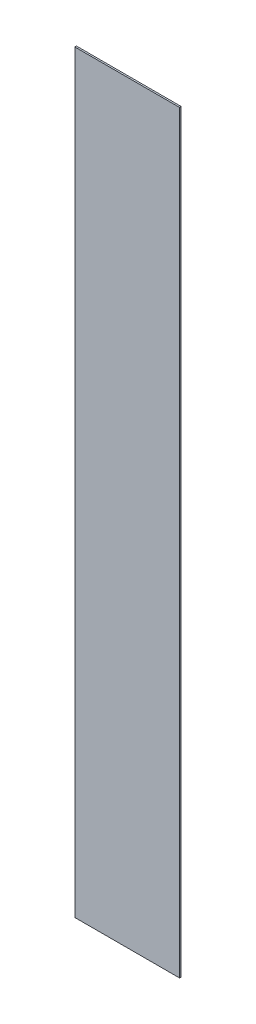
SolidWorks part; units mm, degrees
material "PMMA(有机玻璃)"
ref_plane "前视" through (0, 0, 0) normal (0, 0, 1) x (1, 0, 0)
ref_plane "上视" through (0, 0, 0) normal (0, 1, 0) x (1, 0, 0)
ref_plane "右视" through (0, 0, 0) normal (1, 0, 0) x (0, 0, -1)
sketch "草图1" plane through (0, 0, 0) normal (0, 0, 1) x (1, 0, 0)
  line L1 (-160.5, 1155) -> (160.5, 1155)
  line L2 (-160.5, 1155) -> (-160.5, -1155)
  line L3 (-160.5, -1155) -> (160.5, -1155)
  line L4 (160.5, 1155) -> (160.5, -1155)
  line L5 (-160.5, 1155) -> (160.5, -1155) construction
  line L6 (-160.5, -1155) -> (160.5, 1155) construction
  point P0 (0, 0)
  dimension "D1" = 2310
  dimension "D2" = 321
extrude "凸台-拉伸1" add sketch "草图1" along normal blind 5
hole_wizard "M5 间隙孔1" positions "草图3" profile "草图2" hole size "M5" standard "GB"
sketch "草图3" plane through (0, 0, 5) normal (0, 0, 1) x (1, 0, 0)
  line L0 (-427.5, 273) -> (-427.5, -273) construction
  line L1 (-427.5, -273) -> (427.5, -273) construction
  line L2 (0, 273) -> (0, -273) construction
  line L3 (427.5, 273) -> (-427.5, 273) construction
  line L5 (-427.5, 0) -> (427.5, 0) construction
  line L6 (427.5, -273) -> (427.5, 273) construction
  point P0 (-375, -261)
  point P46 (415.5, 250)
  point P48 (-415.5, 250)
  point P58 (-125, -261)
  point P59 (125, -261)
  point P61 (-125, 261)
  point P62 (125, 261)
  point P64 (-375, 261)
  point P88 (375, -261)
  point P89 (375, 261)
  point P108 (415.5, 0)
  point P109 (-415.5, 0)
  point P110 (415.5, -250)
  point P111 (-415.5, -250)
  dimension "D1" = 12
  dimension "D2" = 12
  dimension "D5" = 3
  dimension "D3" = 12
  dimension "D6" = 4
  dimension "D4" = 2
sketch "草图2" plane through (-375, -261, 5) normal (1, 0, 0) x (0, -1, 0)
  line L0 (0, 0) -> (0, 5)
  line L1 (0, 5) -> (2.75, 5)
  line L2 (2.75, 5) -> (2.75, 0)
  line L5 (2.75, 0) -> (0, 0)
  line L11 (0, -6.35) -> (0, 107.95) construction
  dimension "通孔孔直径" = 5.5
  dimension "通孔孔深度" = 5
